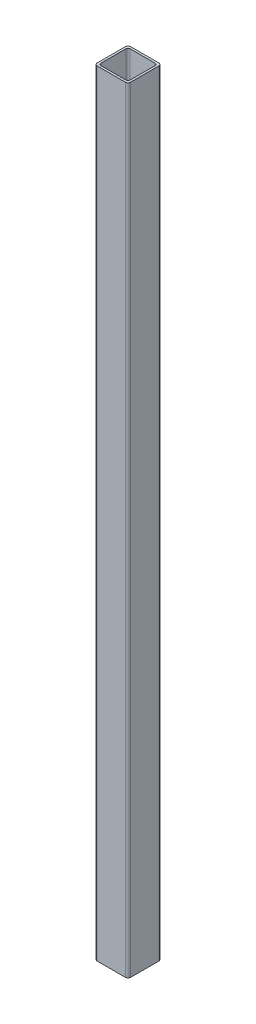
from build123d import *

# Parameters (mm, degrees)
BOSS_EXTRUDE1_DEPTH = 2320


with BuildPart() as part:
    # Sketch2 → Boss-Extrude1 (new body)
    with BuildSketch(Plane(origin=(0, 0, 0), x_dir=(1, 0, 0), z_dir=(0, 1, 0))):
        with BuildLine():
            Line((7.875, -1.525), (92.125, -1.525))
            ThreePointArc((92.125, -1.525), (97.693465902, 0.781534098), (100, 6.35))
            Line((100, 6.35), (100, 90.6))
            ThreePointArc((100, 90.6), (97.693465902, 96.168465902), (92.125, 98.475))
            Line((92.125, 98.475), (7.875, 98.475))
            ThreePointArc((7.875, 98.475), (2.306534098, 96.168465902), (0, 90.6))
            Line((0, 90.6), (0, 6.35))
            ThreePointArc((0, 6.35), (2.306534098, 0.781534098), (7.875, -1.525))
        make_face()
        with BuildLine():
            Line((12.6, 4.775), (87.4, 4.775))
            ThreePointArc((87.4, 4.775), (91.854772721, 6.620227279), (93.7, 11.075))
            Line((93.7, 11.075), (93.7, 85.875))
            ThreePointArc((93.7, 85.875), (91.854772721, 90.329772721), (87.4, 92.175))
            Line((87.4, 92.175), (12.6, 92.175))
            ThreePointArc((12.6, 92.175), (8.145227279, 90.329772721), (6.3, 85.875))
            Line((6.3, 85.875), (6.3, 11.075))
            ThreePointArc((6.3, 11.075), (8.145227279, 6.620227279), (12.6, 4.775))
        make_face(mode=Mode.SUBTRACT)
    extrude(amount=BOSS_EXTRUDE1_DEPTH)


solid = part.part
